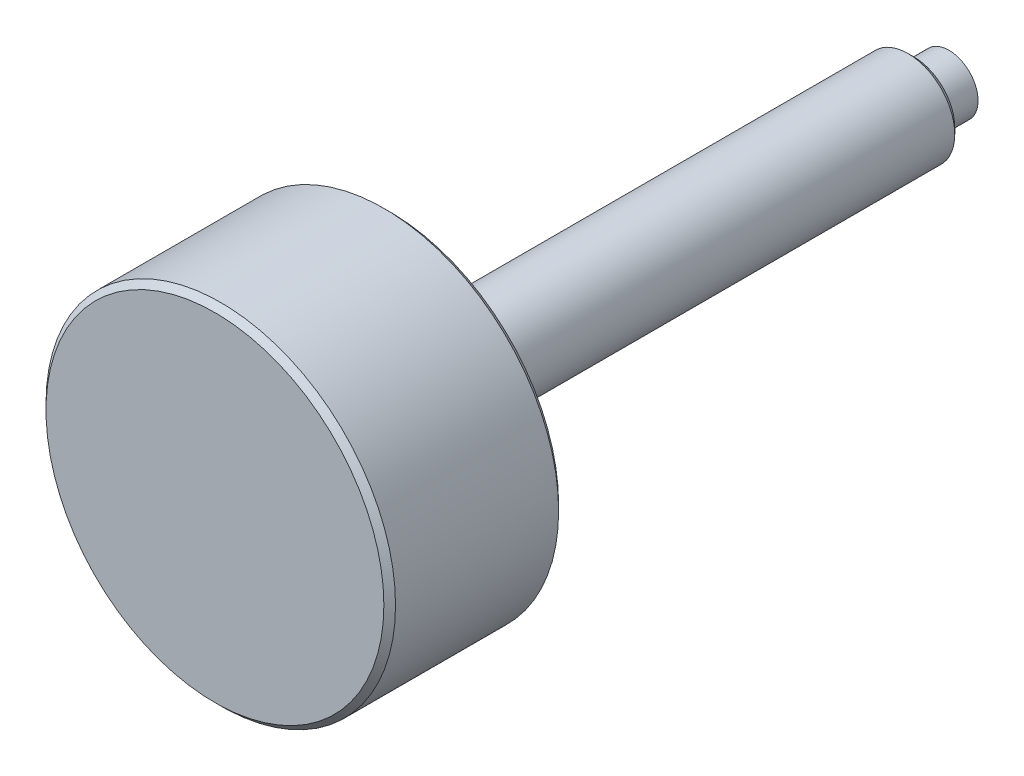
from build123d import *

# Parameters (mm, degrees)
SKETCH1_R           = 4
BOSS_EXTRUDE1_DEPTH = 45
SKETCH2_R           = 15
BOSS_EXTRUDE2_DEPTH = 15
SKETCH3_R           = 2.5
CUT_EXTRUDE1_DEPTH  = 4
SKETCH4_R           = 2.5
BOSS_EXTRUDE3_DEPTH = 7
CHAMFER1_SIZE       = 0.5


with BuildPart() as part:
    # Sketch1 → Boss-Extrude1 (new body)
    with BuildSketch(Plane.XY):
        with Locations(Location((0, 0, 0), (0, 0, 180))):
            Circle(SKETCH1_R)
    extrude(amount=BOSS_EXTRUDE1_DEPTH)

    # Sketch2 → Boss-Extrude2 (add)
    with BuildSketch(Plane.XY.offset(45)):
        Circle(SKETCH2_R)
    extrude(amount=BOSS_EXTRUDE2_DEPTH)

    # Sketch3 → Cut-Extrude1 (cut)
    with BuildSketch(Plane(origin=(0, 0, 0), x_dir=(-1, 0, 0), z_dir=(0, 0, -1))):
        Circle(SKETCH3_R)
    extrude(amount=-CUT_EXTRUDE1_DEPTH, mode=Mode.SUBTRACT)

    # Chamfer1
    chamfer1_edges = [part.edges().sort_by_distance(p)[0] for p in [
        (4, 0, 0),
        (-15, 0, 45),
        (-15, 0, 60),
    ]]
    chamfer(chamfer1_edges, length=CHAMFER1_SIZE)


with BuildPart() as body_2:
    # Sketch4 → Boss-Extrude3 (new body)
    with BuildSketch(Plane(origin=(0, 0, 4), x_dir=(-1, 0, 0), z_dir=(0, 0, -1))):
        Circle(SKETCH4_R)
    extrude(amount=BOSS_EXTRUDE3_DEPTH)


solid = Compound([part.part, body_2.part])
